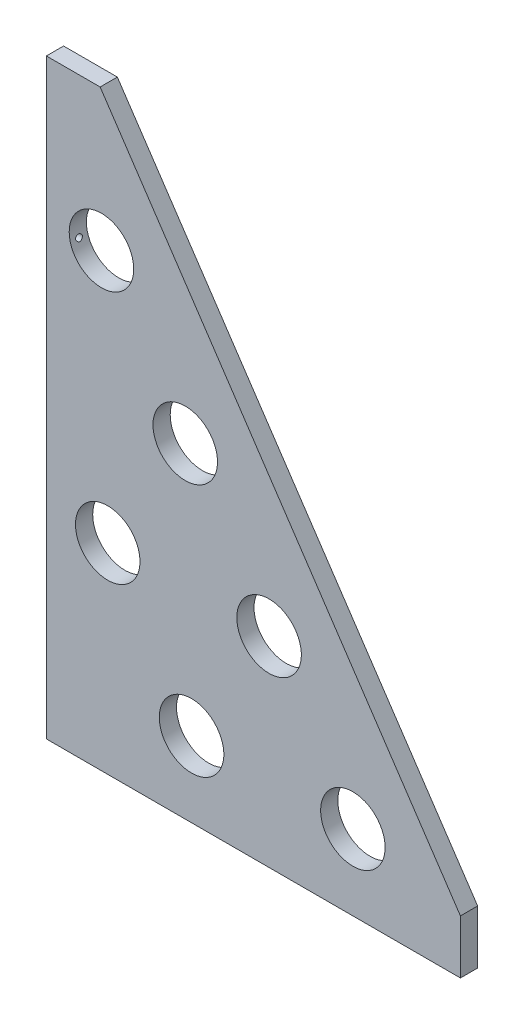
from build123d import *

# Parameters (mm, degrees)
EXTRUDE_1_DEPTH        = 8
PATTERN_LINEAR_1_COUNT = 10
PATTERN_LINEAR_1_PITCH = 55
PATTERN_LINEAR_2_COUNT = 8
PATTERN_LINEAR_2_PITCH = 50
SKETCH_6_R             = 30
CUT_EXTRUDE_1_DEPTH    = 672.551189411


with BuildPart() as part:
    # 草图1 → 凸台-拉伸1 (new, symmetric)
    with BuildSketch(Plane.XY):
        Polygon((0, 0), (385, 0), (385, 50), (50, 550), (0, 550), align=None)
    extrude(amount=EXTRUDE_1_DEPTH, both=True)

    # 草图3 → M8 螺纹孔1 (revolve, cut)
    with BuildSketch(Plane.ZX.offset(520)):
        Polygon((0, 0), (0, 24.292926105), (3.4, 22.25), (3.4, 0), align=None)
    hole_wizard_m8_1 = revolve(axis=Axis((-6.35, 520, 0), (1, 0, 0)), mode=Mode.SUBTRACT)

    # 阵列(线性)1: M8 螺纹孔1 ×10
    with Locations(*[(0, -i * PATTERN_LINEAR_1_PITCH, 0) for i in range(1, PATTERN_LINEAR_1_COUNT)]):
        add(hole_wizard_m8_1, mode=Mode.SUBTRACT)

    # 草图5 → M8 螺纹孔2 (revolve, cut)
    with BuildSketch(Plane(origin=(20, 0, 0), x_dir=(0, 0, -1), z_dir=(1, 0, 0))):
        Polygon((0, 0), (0, 24.292926105), (3.4, 22.25), (3.4, 0), align=None)
    hole_wizard_m8_2 = revolve(axis=Axis((20, -6.35, 0), (0, 1, 0)), mode=Mode.SUBTRACT)

    # 阵列(线性)2: M8 螺纹孔2 ×8
    with Locations(*[(i * PATTERN_LINEAR_2_PITCH, 0, 0) for i in range(1, PATTERN_LINEAR_2_COUNT)]):
        add(hole_wizard_m8_2, mode=Mode.SUBTRACT)

    # 草图6 → 切除-拉伸1 (cut, through all)
    with BuildSketch(Plane(origin=(0, 0, -8), x_dir=(-1, 0, 0), z_dir=(0, 0, -1))):
        with Locations((-285, 70)):
            Circle(SKETCH_6_R)
        with Locations((-129.147552133, 302.615593832)):
            Circle(SKETCH_6_R)
        with Locations((-207.073776066, 186.307796916)):
            Circle(SKETCH_6_R)
        with Locations((-135, 70)):
            Circle(SKETCH_6_R)
        with Locations((-51.221328199, 418.923390748)):
            Circle(SKETCH_6_R)
        with Locations((-57.073776066, 186.307796916)):
            Circle(SKETCH_6_R)
    extrude(amount=-CUT_EXTRUDE_1_DEPTH, mode=Mode.SUBTRACT)


solid = part.part
